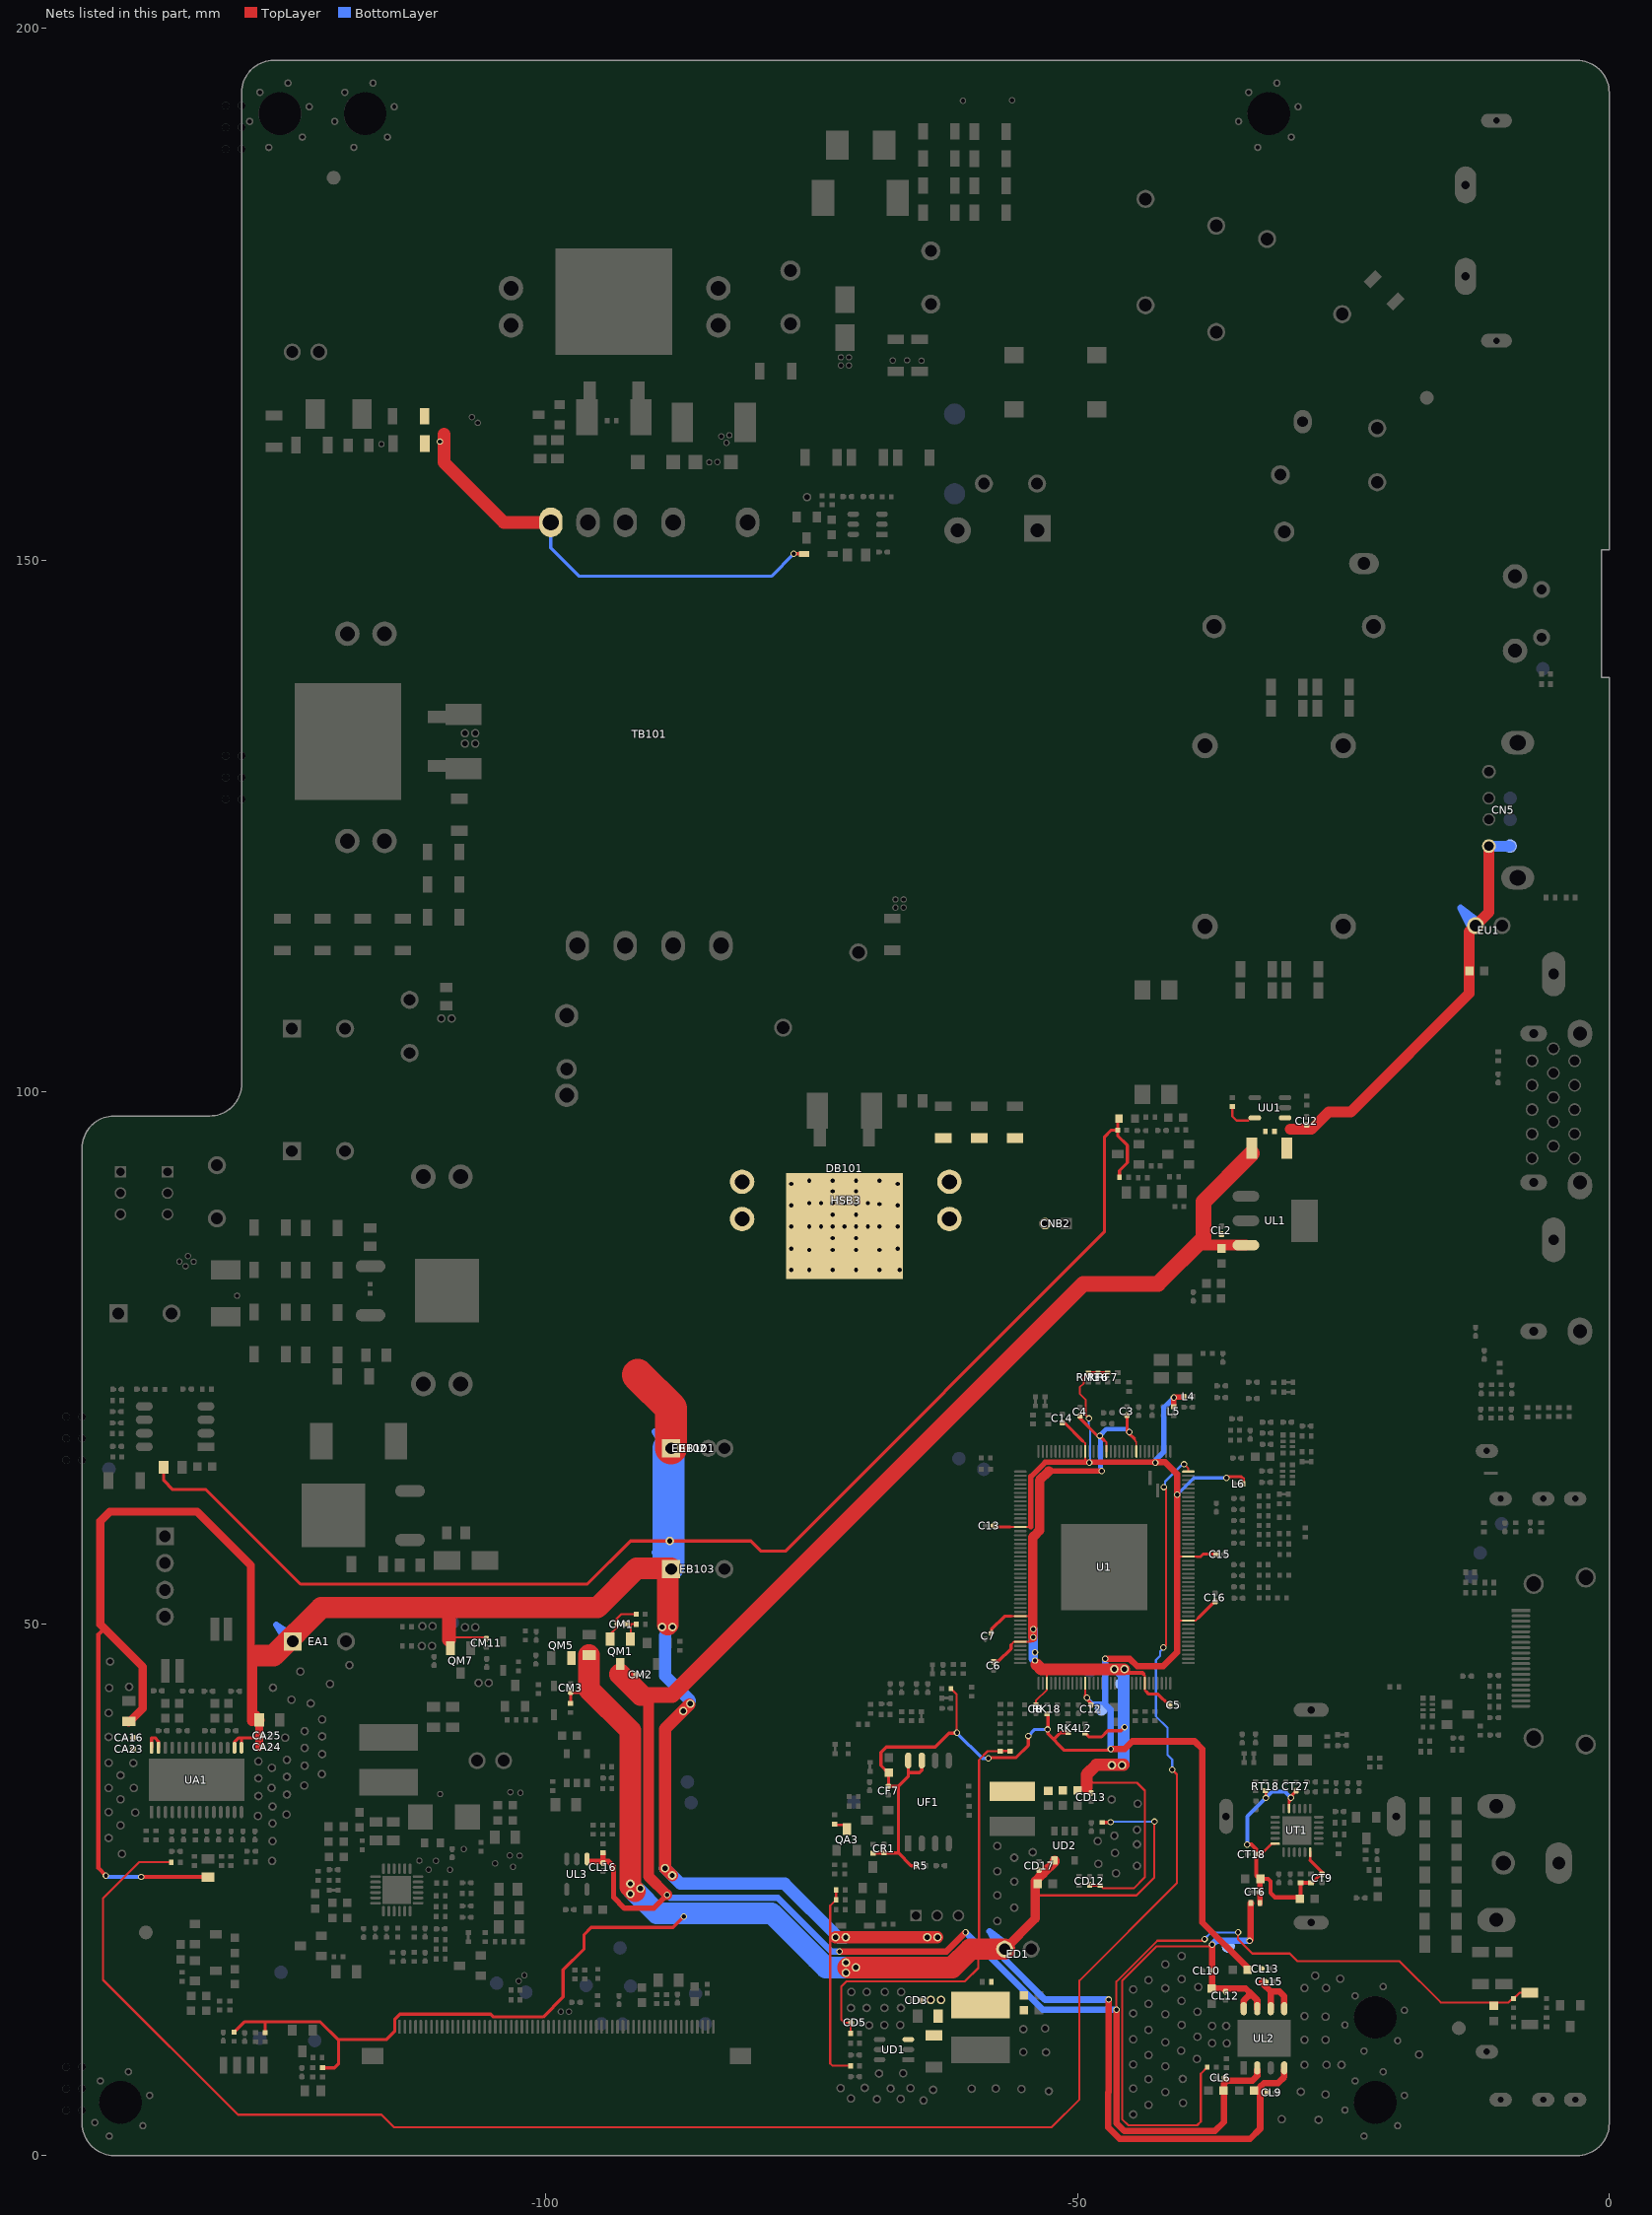
[diagram p0: the nets of this part, all layers, seen from the top]
# Altium PCB MISC86383-9.PcbDoc (part 7 of 18)
Units mm, origin at the board's own origin, x right, y up, seen from the top; angles counter-clockwise.
Board outline 143.6 x 197 mm, 2 copper layers (TopLayer, BottomLayer), stack 1.571 mm thick; 743 components, 401 nets, 2996 pads, 1077 vias.
Unrouted connection lines stored in the file: 4.

## Free pads (board coordinates)
  round 4 on Keep-Out: 0(-268.7,5) 0(-5,192)
  oval 5x4 on Keep-Out: 0(-258.2,192) 0(-15.5,5)
  round 0.7 hole 0.7 unplated: VIA5(-145.1,4.25) VIA5(-145.1,6.29) VIA5(-145.1,8.33) VIA5(-145.1,65.385) VIA5(-145.1,67.425) VIA5(-145.1,69.465) VIA5(-143.6,4.25) VIA5(-143.6,6.29) VIA5(-143.6,8.33) VIA5(-143.6,65.385) VIA5(-143.6,67.425) VIA5(-143.6,69.465) VIA5(-130.1,127.535) VIA5(-130.1,129.575) VIA5(-130.1,131.615) VIA5(-130.1,188.67) VIA5(-130.1,190.71) VIA5(-130.1,192.75) VIA5(-128.6,127.535) VIA5(-128.6,131.615) VIA5(-128.6,188.67) VIA5(-128.6,190.71) VIA5(-128.6,192.75) VIA5(-128.6,129.575)
  round 0.8 hole 0.5 paste-0.4 mask-0.4: VIA5(-141.108,29.858) VIA5(-141.108,32.293) VIA5(-141.108,34.55) VIA5(-141.108,36.923) VIA5(-141.108,39.359) VIA5(-141.108,41.616) VIA5(-141.051,43.962) VIA5(-140.972,46.448) VIA5(-139.985,31.058) VIA5(-139.985,33.494) VIA5(-139.985,35.751) VIA5(-139.865,28.364) VIA5(-139.183,44.072) VIA5(-138.789,36.901) VIA5(-138.736,34.561) VIA5(-138.613,32.249) VIA5(-127.075,31.927) VIA5(-127.036,33.802) VIA5(-127.036,35.472) VIA5(-127.036,37.052) VIA5(-125.789,34.571) VIA5(-125.75,36.447) VIA5(-125.739,27.698) VIA5(-125.699,29.573) VIA5(-125.699,31.242) VIA5(-125.699,32.822) VIA5(-125.654,43.993) VIA5(-124.511,39.281) VIA5(-124.388,32.068) VIA5(-124.349,33.943) VIA5(-124.349,35.612) VIA5(-124.349,37.192) VIA5(-123.916,42.859) VIA5(-123.084,45.51) VIA5(-122.72,34.782) VIA5(-122.68,36.657) VIA5(-122.68,38.326) VIA5(-122.68,39.907) VIA5(-122.117,42.511) VIA5(-121.062,35.866) VIA5(-121.022,37.741) VIA5(-121.022,39.41) VIA5(-121.022,40.991) VIA5(-120.288,44.34) VIA5(-118.466,46.106) VIA5(-111.658,47.904) VIA5(-111.608,49.784) VIA5(-110.693,47.904) VIA5(-110.642,49.784) VIA5(-109.83,106.921) VIA5(-108.864,106.921) VIA5(-107.607,132.766) VIA5(-107.607,133.731) VIA5(-107.594,49.67) VIA5(-106.642,132.766) VIA5(-106.642,133.731) VIA5(-106.629,49.67) VIA5(-106.324,44.45) VIA5(-105.359,44.45) VIA5(-92.05,24.587) VIA5(-92.05,25.552) VIA5(-91.11,25.095) VIA5(-89.065,49.695) VIA5(-88.794,27.021) VIA5(-88.341,57.785) VIA5(-88.111,26.338) VIA5(-88.1,49.695) VIA5(-87.084,41.796) VIA5(-86.401,42.478) VIA5(-75.425,155.943) VIA5(-72.758,20.523) VIA5(-72.268,6.335) VIA5(-71.793,20.523) VIA5(-71.78,17.17) VIA5(-71.78,18.136) VIA5(-71.305,5.352) VIA5(-71.301,13.875) VIA5(-71.279,15.377) VIA5(-70.841,17.678) VIA5(-70.01,6.361) VIA5(-69.836,13.875) VIA5(-69.814,15.377) VIA5(-69.592,12.245) VIA5(-68.869,5.301) VIA5(-68.653,7.709) VIA5(-68.17,12.263) VIA5(-68.15,13.875) VIA5(-68.128,15.377) VIA5(-67.575,6.31) VIA5(-66.663,12.263) VIA5(-66.612,5.327) VIA5(-66.608,13.875) VIA5(-66.586,15.377) VIA5(-66.396,7.734) VIA5(-65.709,6.332) VIA5(-64.478,5.173) VIA5(-64.135,20.523) VIA5(-63.805,14.63) VIA5(-63.574,6.178) VIA5(-63.17,20.523) VIA5(-62.84,14.63) VIA5(-59.95,6.275) VIA5(-57.692,6.301) VIA5(-57.541,22.035) VIA5(-57.541,24.471) VIA5(-57.541,26.728) VIA5(-57.541,29.101) VIA5(-55.947,23.314) VIA5(-55.947,25.749) VIA5(-55.947,28.006) VIA5(-55.257,6.25) VIA5(-55.103,9.738) VIA5(-55.09,11.88) VIA5(-54.216,28.516) VIA5(-53.042,11.949) VIA5(-52.967,9.703) VIA5(-52.697,6.041) VIA5(-48.108,29.566) VIA5(-48.032,27.427) VIA5(-46.787,33.477) VIA5(-46.768,36.697) VIA5(-46.535,45.744) VIA5(-46.533,30.074) VIA5(-46.482,28.448) VIA5(-46.384,26.536) VIA5(-45.803,36.697) VIA5(-45.57,45.744) VIA5(-44.77,3.862) VIA5(-44.77,6.298) VIA5(-44.77,8.555) VIA5(-44.77,10.928) VIA5(-44.77,13.363) VIA5(-44.77,15.62) VIA5(-44.405,27.228) VIA5(-44.405,29.26) VIA5(-44.405,30.632) VIA5(-44.351,33.07) VIA5(-43.326,4.747) VIA5(-43.326,7.183) VIA5(-43.326,9.44) VIA5(-43.326,11.813) VIA5(-43.326,14.248) VIA5(-43.326,16.505) VIA5(-41.739,5.956) VIA5(-41.739,8.392) VIA5(-41.739,10.649) VIA5(-41.739,13.286) VIA5(-41.739,15.722) VIA5(-41.739,17.979) VIA5(-40.254,9.848) VIA5(-40.228,14.541) VIA5(-40.208,18.748) VIA5(-40.203,12.284) VIA5(-40.195,16.592) VIA5(-40.098,7.201) VIA5(-40.073,4.944) VIA5(-38.766,9.081) VIA5(-38.71,11.176) VIA5(-38.71,13.513) VIA5(-38.645,15.833) VIA5(-37.338,10.566) VIA5(-37.338,12.192) VIA5(-36.017,12.192) VIA5(-35.966,10.54) VIA5(-30.785,3.404) VIA5(-29,5.994) VIA5(-28.651,8.534) VIA5(-28.651,10.871) VIA5(-28.651,13.106) VIA5(-28.651,15.748) VIA5(-27.635,16.916) VIA5(-27.33,3.353) VIA5(-26.67,5.74) VIA5(-26.67,10.871) VIA5(-26.67,13.056) VIA5(-26.619,15.748) VIA5(-26.568,8.534) VIA5(-25.298,16.612) VIA5(-25.171,8.522) VIA5(-17.882,9.5)
  round 0.6 hole 0.4 paste-0.4 mask-0.4: VIA5(-134.455,84.061) VIA5(-133.871,83.617) VIA5(-133.655,84.582) VIA5(-133.116,84.043) VIA5(-129.032,80.848) VIA5(-115.456,160.922) VIA5(-111.887,27.724) VIA5(-111.014,26.873) VIA5(-110.325,27.711) VIA5(-109.957,161.163) VIA5(-109.931,33.985) VIA5(-109.004,26.86) VIA5(-107.709,28.816) VIA5(-106.94,163.468) VIA5(-106.402,162.929) VIA5(-104.762,27.47) VIA5(-103.391,28.219) VIA5(-103.327,34.163) VIA5(-103.083,27.14) VIA5(-102.552,16.408) VIA5(-102.464,28.194) VIA5(-102.387,34.112) VIA5(-102.014,16.947) VIA5(-98.59,13.525) VIA5(-97.828,13.525) VIA5(-84.633,159.22) VIA5(-83.858,159.245) VIA5(-83.49,161.658) VIA5(-83.007,161.049) VIA5(-82.74,161.76) VIA5(-72.25,168.326) VIA5(-72.25,169.088) VIA5(-71.488,168.326) VIA5(-71.488,169.088) VIA5(-67.373,168.796) VIA5(-67.119,117.348) VIA5(-67.119,118.11) VIA5(-66.357,117.348) VIA5(-66.357,118.11) VIA5(-66.015,168.808) VIA5(-64.668,168.77) VIA5(-60.769,193.218) VIA5(-56.147,193.256) VIA5(-54.15,48.733) VIA5(-54.15,49.495) VIA5(-53.994,46.545) VIA5(-53.994,47.307)

## Via types
v1: diameter 0.6, hole 0.4, TopLayer to BottomLayer, tented both sides, 993 vias
v2: diameter 0.6, hole 0.4, TopLayer to BottomLayer, 65 vias
v3: diameter 0.7, hole 0.5, TopLayer to BottomLayer, tented both sides, 15 vias
v4: diameter 0.8, hole 0.5, TopLayer to BottomLayer, tented both sides, 4 vias

## Nets (pads, with @x,y where several pads share a name; then routed paths per layer and width w, separated by ;. In a path a pad name is that pad's centre, name@x,y a point inside that pad or via, vN(x,y) a via of type N, cw(c..) or ccw(c..) an arc to the next point about the centre after c; other vN are vias at no path point)
1.15V_STB: 1.15V_STB.1 C3.2@-45.337,69.569 C3.2@-45.337,69.744 C4.2@-49.757,69.68 C4.2@-49.757,69.505 C5.2@-41.206,42.333 C5.2@-41.381,42.333 C6.2@-57.891,46.297 C6.2@-57.891,46.472 C7.2@-58.079,49.149 C7.2@-58.203,49.025 C8.2@-53.91,42.228 C8.2@-53.91,42.403 CD10.2 CD12.2@-48.854,25.57 CD12.2@-48.854,25.395 CD13.2@-48.717,33.943 CD13.2@-48.717,34.118 CD14.2 CD15.2 L2.1 LD2.1 pad.VIA5@-45.57,45.744 pad.VIA5@-45.803,36.697 pad.VIA5@-46.535,45.744 pad.VIA5@-46.768,36.697 pad.VIA5@-53.994,46.545 pad.VIA5@-53.994,47.307 pad.VIA5@-54.15,48.733 pad.VIA5@-54.15,49.495 RD9.1 U1.55 U1.62 U1.113 U1.119 U1.127 U1.150 | length 103.6
  TopLayer w0.178: -56.259,48 -55.947,48.313 -54.344,48.313 ; -56.246,50.715 -56.244,50.713 -54.199,50.713 ; C8.2@-53.91,42.403 -53.91,42.749 -52.871,43.788 -52.871,45.343 ; -47.458,67.251 -47.271,67.063 U1.62@-47.271,66.213 ; -44.661,67.311 -44.471,67.121 U1.55@-44.471,66.213 ; -43.811,45.303 -43.671,45.163 -43.671,43.758 -43.518,43.605
  TopLayer w0.203: CD15.2@-51.372,34.33 CD15.2@-51.318,34.383 ; CD10.2@-49.974,34.323 CD10.2@-49.947,34.296 ; CD12.2@-48.854,25.395 RD9.1@-47.865,25.395 -47.591,25.121 -44.717,25.121 -43.663,26.175 -43.663,34.315 -44.399,35.052 -48.565,35.052 -48.768,35.255
  TopLayer w0.305: C7.2@-58.079,49.149 -58.079,49.495 -56.859,50.715 -56.246,50.715 ; C6.2@-57.891,46.472 -57.437,46.472 -56.259,47.65 -56.259,48 ; C4.2@-49.757,69.505 -49.757,69.312 v1@-48.112,67.667 ; L2.1@-49.122,39.552 -48.931,39.361 -47.734,39.361 -47.163,39.933 -45.919,39.933 v1(-45.568,40.284) ; v1@-47.918,67.667 -47.502,67.251 ; -45.337,69.162 C3.2@-45.337,69.569 ; -45.336,69.268 -45.336,68.068 v1@-45.206,67.938 ; v1(-45.11,68.034) v1@-45.206,67.938 ; -44.629,67.361 v1@-45.206,67.938 ; -43.518,43.605 -43.3,43.387 -42.435,43.387 C5.2@-41.381,42.333
  TopLayer w0.381: pad.VIA5@-45.629,45.711 -45.615,45.698 -45.302,45.384 -43.892,45.384 -43.811,45.303
  TopLayer w0.508: -52.699,64.36 v1(-47.725,64.36)
  TopLayer w0.889: pad.VIA5@-54.199,48.683 -54.199,48.733 -54.199,49.495 -54.199,50.713 -54.199,58.173 -54.085,58.287 -54.048,58.287 -53.564,58.771 -53.564,59.364 -53.564,63.495 -52.699,64.36
  TopLayer w1.143: -53.841,46.162 -53.39,45.711 -46.535,45.711 pad.VIA5@-45.629,45.711 ; -49.136,34.604 -49.136,35.827 -48.222,36.741 -46.768,36.741 -45.803,36.741 pad.VIA5@-45.663,36.741
  BottomLayer w0.457: v1(-47.725,64.36) -47.826,64.462 -47.826,67.674 -47.826,67.772 -47.293,68.305 -45.382,68.305 v1(-45.11,68.034)
  BottomLayer w0.889: pad.VIA5@-54.15,46.701 -54.15,47.307 pad.VIA5@-54.15,48.733 pad.VIA5@-54.15,49.495
  BottomLayer w1.143: -45.923,45.466 -45.885,45.428 -45.663,45.205 -45.663,44.348 -45.663,40.284 pad.VIA5@-45.663,36.785
  other v1: -47.911,67.674
3V3_STB: 3V3_STB.1 C12.2@-48.728,42.228 C12.2@-48.728,42.403 C13.2@-57.853,59.212 C13.2@-58.028,59.212 C14.2@-51.435,68.885 C14.2@-51.435,69.06 C15.2@-36.826,56.54 C15.2@-37.001,56.54 C16.2@-37.059,52.051 C16.2@-37.059,52.226 CF7.1 CF10.2 CL13.1 CL14.1 CL15.1 CR1.2@-68.191,28.441 CR1.2@-68.191,28.616 L4.1 L5.1 L6.1 R5.2 RF6.2 RF7.2 RF14.1 RK4.2 RK18.2 RM3.1 RR5.2 U1.11 U1.26 U1.67 U1.92 U1.136 UF1.7 UF1.8 UL2.5 UL2.6 | length 190.8
  TopLayer w0.178: -56.348,59.11 -56.345,59.113 -54.412,59.113 ; -49.505,67.183 -49.271,66.949 U1.67@-49.271,66.213 -49.271,65.292 ; -49.271,43.32 U1.136@-49.271,44.413 ; RM3.1@-48.969,73.581 -48.987,73.581 -49.41,73.158 -49.41,72.631 -49.785,72.256 -49.785,71.636 -49.206,71.057 -49.206,69.58 v1(-48.93,69.305) ; -40.617,50.313 U1.11@-39.571,50.313 -38.881,50.313 -38.653,50.541 ; -40.371,56.313 -38.768,56.313
  TopLayer w0.203: RF14.1@-61.907,43.901 -61.366,43.361 -61.366,39.776 -61.341,39.751 v1@-61.328,39.738
  TopLayer w0.254: -38.768,56.313 -38.412,56.313 -38.17,56.555 C15.2@-37.076,56.555
  TopLayer w0.305: RR5.2@-69.207,28.415 -68.216,28.415 CR1.2@-68.191,28.441 -66.893,28.441 ; UF1.8@-65.916,37.142 -65.916,35.965 ; R5.2@-65.137,27.254 -65.636,27.254 -66.858,28.476 -66.84,28.494 -66.84,34.688 ; UF1.7@-64.646,37.142 -64.632,37.128 -64.632,36.215 -64.853,35.994 -65.887,35.994 -65.916,35.965 ; v1@-61.328,39.738 -61.29,39.7 -61.328,39.7 -62.078,39.7 -63.378,38.4 -67.988,38.4 -68.484,37.904 -68.484,36.672 -67.787,35.975 -67.778,35.975 CF10.2@-67.755,35.997 -67.755,34.749 CF7.1@-67.783,34.721 -66.873,34.721 -66.84,34.688 ; v1(-58.369,37.338) -58.445,37.414 -58.369,37.414 -55.778,37.414 -54.62,38.572 v1(-54.62,39.45) ; C13.2@-57.853,59.212 -57.752,59.11 -56.348,59.11 ; RK18.2@-52.779,41.527 -52.779,40.059 -52.779,39.643 -51.24,38.104 v1@-47.088,38.104 ; -52.195,39.158 -51.592,39.762 RK4.2@-50.874,39.762 ; C14.2@-51.435,68.885 -51.201,68.885 -49.505,67.188 -49.505,67.183 ; v1@-49.249,43.298 -49.249,43.056 -49.186,42.994 -48.728,42.536 C12.2@-48.728,42.403 C12.2@-48.728,42.228 ; RM3.1@-48.901,73.593 RF6.2@-48.062,73.593 RF7.2@-47.147,73.593 RF7.2@-47.071,73.593 ; C12.2@-48.713,42.417 C12.2@-48.688,42.392 ; C12.2@-48.677,42.228 C12.2@-48.677,42.381 ; -38.653,50.541 -37.143,52.051 C16.2@-37.059,52.051 ; v1@-35.956,63.68 v1(-36.005,63.729) -35.903,63.83 -34.595,63.83 -34.385,63.62 L6.1@-34.385,63.17 ; -66.84,34.688 -65.916,35.613 -65.916,35.965
  TopLayer w0.508: -54.39,59.113 -54.39,63.837 -53.041,65.185 -48.893,65.185 v1@-42.784,65.185 ; L5.1@-40.959,70.58 -40.959,71.235 v1(-40.93,71.264) -40.895,71.299 -40.191,71.299 L4.1@-40.164,71.326
  TopLayer w0.61: v1(-47.401,46.715) -45.093,46.715 -44.385,46.007 -41.951,46.007 -40.628,47.329 -40.628,62.154 -40.628,64.066 -41.743,65.181 -42.683,65.181 v1@-42.784,65.181 ; v1@-46.863,38.231 -45.562,38.231 -44.851,38.942 -38.979,38.942 -38.259,38.222 -38.259,21.921 -33.99,17.652 CL14.1@-33.99,17.475 ; -32.66,16.358 -32.66,16.251 -32.572,16.164 -32.485,16.076 -31.826,15.418 ; UL2.6@-31.826,13.806 -31.826,15.418 ; UL2.5@-30.556,13.806 -30.556,14.961 -31.013,15.418 -31.826,15.418
  BottomLayer w0.178: v1(-48.93,69.305) -48.93,68.488 -48.792,68.35 v1@-48.792,65.257
  BottomLayer w0.305: v1@-61.341,39.726 -58.953,37.338 v1(-58.369,37.338) ; v1(-54.62,39.45) -54.012,40.059 v1(-52.806,40.059) ; v1(-49.123,43.056) -48.608,42.541 -47.752,42.541 3V3_STB.1@-47.511,42.541 ; v1(-40.64,62.154) -39.065,63.729 v1(-36.005,63.729)
  BottomLayer w0.508: v1(-42.683,65.155) -42.683,65.371 -41.862,66.192 -41.862,70.332 v1(-40.93,71.264)
  BottomLayer w0.61: v1@-47.387,46.7 v1(-47.401,46.715) -47.401,42.431 -47.367,42.397 -46.888,41.918 -46.888,38.227 -46.876,38.214 -46.863,38.202 v1(-46.863,38.227)
  other v1: -61.328,39.764 -48.893,65.155
3V3_TUN: CT2.2 CT5.2 CT6.1 CT9.1 CT18.2@-33.189,28.323 CT18.2@-33.364,28.323 CT27.1 LT1.1 LT2.2 LT12.2 RT18.1 UT1.11 UT1.18 UT1.24 | length 30.2
  TopLayer w0.203: RT18.1@-32.344,34.299 -32.293,34.248 v1(-32.293,33.619) ; UT1.11@-30.11,32.62 -30.11,33.263 -30.071,33.301
  TopLayer w0.229: CT18.2@-33.189,28.323 -32.741,28.323 -31.744,29.32 UT1.18@-31.41,29.32 ; UT1.24@-28.11,28.52 -28.11,27.771 -28.102,27.764
  TopLayer w0.305: -30.071,33.301 -30.071,33.638 -29.998,33.711 v1@-29.931,33.778 ; v1(-29.931,33.644) v1@-29.931,33.778 ; CT27.1@-29.436,34.273 v1@-29.931,33.778 ; -28.102,27.764 CT9.1@-26.997,26.659 ; LT1.1@-27.922,25.638 -27.122,26.437 CT9.1@-27.072,26.487
  TopLayer w0.381: v1(-34.033,29.245) -33.647,29.245 -33.189,28.787 CT18.2@-33.189,28.323 -33.189,26.314 -32.887,26.012 -32.838,26.012 CT5.2@-32.811,26.012 -32.065,26.012 -31.836,25.783 -31.836,24.691 -31.421,24.277 -29.302,24.277 -29.27,24.309 -29.029,24.549 LT2.2@-29.029,25.638 LT1.1@-28.064,25.638 LT1.1@-27.922,25.638 ; CT9.1@-27.072,26.487 CT9.1@-26.997,26.487
  TopLayer w0.508: LT12.2@-32.838,23.726 -32.838,24.767 CT5.2@-32.838,26.012
  BottomLayer w0.381: v1(-34.033,29.245) -34.033,31.88 v1(-32.293,33.619) -31.689,34.224 -30.511,34.224 v1(-29.931,33.644)
3V3_TUNER: 3V3_TUNER.1 CL10.2@-37.421,17.374 CL10.2@-37.596,17.374 CL11.1 CL12.2@-36.068,15.262 CL12.2@-36.068,15.437 LT12.1 RL5.2 UL2.7 UL2.8 | length 54.7
  TopLayer w0.203: RL5.2@-37.795,8.306 -38.405,7.696 -38.405,3.175 -38.748,2.832 -45.22,2.832 -45.806,3.419 -45.806,16.423 -42.569,19.66 -37.519,19.66 v1(-37.338,19.841)
  TopLayer w0.508: LT12.1@-33.701,23.738 LT12.1@-33.688,23.726
  TopLayer w0.61: v1(-37.338,19.841) -37.338,17.374 -37.338,15.743 CL11.1@-37.389,15.692 -36.068,15.692 -34.184,15.692 -33.706,15.215 ; UL2.8@-34.366,13.806 -34.366,14.554 -33.706,15.215 ; v1(-33.817,20.181) -33.714,20.284 -33.714,23.7 LT12.1@-33.688,23.726 ; UL2.7@-33.096,13.806 -33.096,14.605 -33.706,15.215
  BottomLayer w0.61: v1(-37.338,19.841) -37.33,19.841 -36.99,20.181 -35.82,20.181 v1(-33.817,20.181)
5V_M: CL1.2 CL2.2@-36.449,86.566 CL2.2@-36.449,86.741 CL6.2@-36.3,7.315 CL6.2@-36.125,7.315 CL7.2 CL16.1 CM2.1 CO77.1 F2.1 FU1.2 QM1.D RL50.1 RO2.2 RO6.1 RU4.2 UL1.3 UL2.2 UL3.1 UU1.5 | length 247
  TopLayer w0.203: v1(-46.339,13.705) -46.339,16.356 -42.49,20.206 -38.2,20.206 v1(-38.053,20.353) ; RU4.2@-35.433,98.635 -35.433,97.714 -35.046,97.327 -33.927,97.327 ; v1(-34.899,20.973) -34.899,20.347 -33.551,18.999 -30.033,18.999 -29.296,18.263 -19.699,18.263 -15.828,14.391 -10.846,14.391 -9.465,14.391 -9.051,14.805 -8.992,14.864 RO6.1@-8.992,14.746 -8.425,15.313 RO2.2@-7.468,15.313
  TopLayer w0.508: UL3.1@-96.012,27.648 CL16.1@-94.628,27.648 ; RL50.1@-94.628,28.468 CL16.1@-94.628,27.648 ; CL16.1@-94.615,27.539 -94.628,27.552 CL16.1@-94.628,27.648 ; CL16.1@-94.615,27.648 -94.094,27.648 -93.624,27.178 -93.624,24.282 -92.596,23.254 -89.852,23.254 v1(-88.595,24.511)
  TopLayer w0.61: v1(-72.384,19.177) -62.332,19.177 v1(-60.528,20.98) ; v1(-46.339,13.705) -46.339,3.039 -45.599,2.299 -37.071,2.299 -36.22,3.15 -36.22,6.096 -36.22,6.756 -35.981,6.996 -35.928,7.048 -33.541,7.048 -33.096,7.493 UL2.2@-33.096,8.038
  TopLayer w1.016: -91.078,43.313 -90.33,42.566 -90.33,26.246 v1(-88.595,24.511) ; -38.713,85.598 -36.449,85.598 UL1.3@-34.163,85.598
  TopLayer w1.5: -91.078,43.313 -88.098,43.313 -49.445,81.966 -42.418,81.966 -38.151,86.233 -38.151,89.687 FU1.2@-33.603,94.235
  TopLayer w2.032: -93.003,45.239 -92.262,44.497 -92.174,44.41 -91.078,43.313
  BottomLayer w0.203: v1(-38.053,20.353) -37.433,20.973 v1(-34.899,20.973)
  BottomLayer w0.61: v1(-88.595,24.511) -88.316,24.232 -78.181,24.232 -73.127,19.177 v1(-72.384,19.177) ; v1(-60.528,20.98) -53.264,13.716 v1@-46.339,13.716
5V_MOS_G: CM1.2@-92.65,49.974 CM1.2@-92.475,49.975 QM1.G RM2.2 | length 2.4
  TopLayer w0.203: CM1.2@-92.475,49.975 -91.999,49.975 ; QM1.G@-92.053,48.571 -91.999,48.625 -91.999,49.975 ; RM2.2@-91.484,49.962 -91.497,49.975 -91.999,49.975
5V_STB: 5V_STB.1 CD5.2@-71.169,12.49 CD5.2@-71.344,12.49 CD7.2 CD9.2 CD16.2 CD17.2@-53.619,26.804 CD17.2@-53.619,26.979 CL8.2 CL9.2@-32,5.944 CL9.2@-32.175,5.944 CM1.1 CM3.2@-97.665,43.538 CM3.2@-97.665,43.713 CM5.2 DK6.K ED1.1 LD1.2 pad.VIA5@-70.841,17.678 pad.VIA5@-71.78,17.17 pad.VIA5@-71.78,18.136 pad.VIA5@-91.11,25.095 pad.VIA5@-92.05,24.587 pad.VIA5@-92.05,25.552 QM1.S QM5.S RD3.2 RD7.2 RK1.2 RK13.1 RK15.1 RM1.2 RM5.2 RV12.2 RV13.2 UD2.4 UL2.4 | length 246.9
  TopLayer w0.203: QM1.S@-93.953,48.571 -93.953,48.998 -93.325,49.626 CM1.1@-93.325,49.974 -93.332,49.981 -93.332,50.482 -92.913,50.902 RM1.2@-91.497,50.902 ; RD3.2@-71.343,11.474 CD5.2@-71.344,12.49 -71.926,12.49 -72.212,12.776 -72.212,15.875 -71.704,16.383 -60.579,16.383 -59.334,17.628 -59.334,18.684 -60.056,19.406 -59.258,20.203 -59.258,37.197 -58.444,38.011 -57.277,38.011 RV13.2@-57.277,38.031 ; RV13.2@-57.247,38.04 -56.35,38.04 RV12.2@-56.333,38.04 ; -53.975,24.308 -53.823,24.46 -44.444,24.46 -42.774,26.13 v1(-42.774,31.394)
  TopLayer w0.305: RK13.1@-129.316,11.591 -128.342,12.565 -126.39,12.565 ; RK15.1@-126.39,11.55 -126.39,12.565 ; RK1.2@-121.006,8.248 -119.882,8.248 -119.482,8.649 -119.482,10.846 ; RM5.2@-97.665,42.508 CM3.2@-97.665,43.538 -96.581,43.538 ; v1(-87.008,22.479) -88.041,21.445 -95.722,21.445 -96.406,20.762 -96.406,19.418 -98.369,17.455 -98.369,14.913 -100.251,13.032 -100.677,13.032 -100.681,13.028 -104.914,13.028 -105.172,13.286 -113.737,13.286 -114.195,12.828 -114.195,11.714 -115.012,10.897 -119.431,10.897 -119.482,10.846 ; RD7.2@-47.689,31.322 -46.91,31.322 v1(-46.888,31.344) ; -126.39,12.565 -121.201,12.565 -119.482,10.846
  TopLayer w0.61: v1(-47.076,14.661) -47.076,5.949 -47.097,5.928 -47.097,2.624 -46.035,1.562 -33.769,1.562 -32.817,2.515 -32.817,6.096 -32.817,6.452 -32.461,6.807 -31.14,6.807 -30.556,7.391 UL2.4@-30.556,8.038
  TopLayer w0.889: ED1.1@-56.851,19.406 -53.975,22.281 -53.975,24.308 -53.975,25.552 -53.975,25.781 -53.973,25.783 -53.286,26.47 -53.198,26.558 -52.149,27.607 UD2.4@-52.149,27.757
  TopLayer w2.032: CM5.2@-95.936,47.053 -95.936,43.85 -92.062,39.976 -92.062,25.552 -92.062,25.286 -91.707,24.93 -91.611,24.835 ; -71.552,17.678 pad.VIA5@-70.841,17.678 -61.783,17.678 -60.056,19.406 ED1.1@-56.851,19.406
  BottomLayer w0.203: v1(-46.888,31.344) -46.838,31.394 v1(-42.774,31.394)
  BottomLayer w0.305: v1@-47.016,31.344 v1(-46.888,31.344)
  BottomLayer w0.61: ED1.1@-56.851,19.406 -56.851,18.446 -53.061,14.656 v1@-47.076,14.656
  BottomLayer w2.032: -91.796,25.019 -91.707,24.93 -91.491,24.714 -89.56,22.784 -87.008,22.784 -78.781,22.784 -74.557,18.56 -73.675,17.678 -71.78,17.678 -71.349,17.678
5V_USB: CN5.1@-11.31,123.13 CU1.2 CU2.1 EU1.1 F2.2 FU1.1 USB_5V.1 UU1.1 | length 38.8
  TopLayer w1.016: -30.003,96.502 -28.448,96.502 -27.984,96.502 -27.949,96.537 -26.365,98.12 -24.308,98.12 -13.152,109.276 CU1.2@-13.152,111.379 -13.152,115.072 EU1.1@-12.578,115.646 -11.31,116.915 CN5.1@-11.31,123.13
  BottomLayer w1.016: CN5.1@-11.31,123.13 USB_5V.1@-9.31,123.13
12V: CA16.2@-138.766,39.278 CA16.2@-138.941,39.278 CA23.2@-138.766,38.212 CA23.2@-138.941,38.212 CA24.2@-126.483,38.427 CA24.2@-126.658,38.427 CA25.2@-126.483,39.494 CA25.2@-126.658,39.494 CA31.2 CA32.2 CD1.2 CD2.1 CD3.2@-64.7,14.605 CD3.2@-64.875,14.605 CM11.2@-105.588,48.447 CM11.2@-105.588,48.622 CNB2.2 DB101.2 EA1.1@-123.798,48.336 EB101.1@-88.212,66.497 EB102.1@-88.212,66.497 EB103.1@-88.212,55.143 HSB3.1 HSB3.2 HSB3.3 HSB3.4 pad.VIA5@-62.84,14.63 pad.VIA5@-63.17,20.523 pad.VIA5@-63.805,14.63 pad.VIA5@-64.135,20.523 pad.VIA5@-71.793,20.523 pad.VIA5@-72.758,20.523 pad.VIA5@-86.401,42.478 pad.VIA5@-87.084,41.796 pad.VIA5@-88.1,49.695 pad.VIA5@-88.111,26.338 pad.VIA5@-88.341,57.785 pad.VIA5@-88.794,27.021 pad.VIA5@-89.065,49.695 QM7.S RA3.1 RA16.1 RA19.2 RB128.2 RB129.2 RB131.2 RB135.1 RB158.2 RB165.2 RB816.1 RD1.1 UA1.15 UA1.16 UA1.27 UA1.28 UD1.3 | length 367.1
  TopLayer w0.203: -108.925,48.73 -105.696,48.73 CM11.2@-105.588,48.622 ; RA16.1@-72.705,24.04 -73.254,23.491 -73.254,21.438 -73.254,8.661 -73.027,8.435 RD1.1@-71.345,8.435
  TopLayer w0.254: RA16.1@-72.705,24.04 RA19.2@-72.705,24.98
  TopLayer w0.3: RB816.1@-135.931,64.706 -135.931,63.477 -135.075,62.621 -131.953,62.621 -123.063,53.731 -96.087,53.731 -92.033,57.785 pad.VIA5@-88.341,57.785 -80.705,57.785 -79.747,56.827 -77.473,56.827 -47.473,86.828 -47.473,95.758 -46.812,96.418 RB158.2@-46.221,96.418 ; RB131.2@-46.102,97.511 -46.221,97.392 RB158.2@-46.221,96.418 ; RB135.1@-46.043,91.973 -46.043,92.615 -45.3,93.358 -45.3,94.983 -46.221,95.904 RB158.2@-46.221,96.418
  TopLayer w0.305: UA1.28@-137.07,38.341 -137.07,39.257 -137.092,39.278 -136.761,39.278 -136.42,38.937 UA1.27@-136.42,38.341 ; UA1.16@-129.27,38.341 -129.27,38.863 -128.855,39.278 -128.57,39.278 ; UA1.15@-128.62,38.341 -128.62,39.228 -128.57,39.278 ; -126.945,39.278 -128.57,39.278
  TopLayer w0.381: -141.519,49.559 -142.076,49.002 -142.076,27.021 v1(-141.366,26.311) ; v1(-138.06,26.199) -131.813,26.199 RA3.1@-131.783,26.17
  TopLayer w0.762: CA31.2@-139.238,40.7 -137.904,42.033 -137.904,45.944 -141.519,49.559 -141.886,49.925 -141.886,59.665 -141.009,60.541 -132.779,60.541 -127.724,55.486 -127.724,46.965 -127.622,46.863 ; -126.945,38.414 -126.945,39.278 CA32.2@-126.945,40.955
  TopLayer w1.016: -127.622,40.881 -127.622,46.863 -127.47,47.015 ; CA32.2@-127.338,41.348 CA32.2@-126.945,40.955
  TopLayer w1.143: pad.VIA5@-88.111,26.338 pad.VIA5@-88.794,27.021 -88.794,40.102 pad.VIA5@-86.486,42.409 ; pad.VIA5@-72.758,20.523 pad.VIA5@-71.793,20.523 pad.VIA5@-64.135,20.523 pad.VIA5@-63.17,20.523
  TopLayer w1.27: -127.47,47.015 -127.089,47.015 ; -109.436,51.524 -109.11,51.198 -109.11,48.472
  TopLayer w2.032: -127.089,47.015 -125.603,47.015 -121.094,51.524 -109.436,51.524 -95.136,51.524 -91.44,55.22 -88.25,55.22 -88.519,54.951 -88.519,49.916
  TopLayer w3: -91.351,73.393 -88.212,70.255 EB101.1@-88.212,66.497
  BottomLayer w0.3: EB103.1@-88.212,55.143 EB103.1@-88.212,55.727
  BottomLayer w0.381: v1(-141.366,26.311) -141.254,26.199 v1(-138.06,26.199)
  BottomLayer w1.143: pad.VIA5@-88.794,27.021 pad.VIA5@-88.111,26.338 -87.338,25.565 -77.529,25.565 -72.487,20.523 pad.VIA5@-71.793,20.523 ; -88.786,48.895 -88.786,45.115 pad.VIA5@-86.452,42.781
  BottomLayer w3: EB103.1@-88.466,55.45 -88.466,55.886 EB101.1@-88.466,66.497
  other v1: -76.918,83.261 -75.218,83.26 -73.018,83.261 -70.818,83.261 -68.618,83.261 -66.719,83.261 -75.218,85.161 -73.018,85.161 -70.818,85.161 -68.618,85.161 -76.918,85.261 -66.918,85.261 -73.018,86.261 -70.818,86.261 -76.919,87.361 -75.218,87.361 -74.118,87.361 -73.018,87.361 -71.918,87.361 -70.818,87.361 -69.718,87.361 -68.618,87.361 -66.919,87.361 -73.018,88.461 -70.818,88.461 -76.918,89.361 -66.918,89.361 -70.818,89.461 -68.618,89.461 -75.218,89.561 -74.119,89.561 -73.018,89.561 -71.918,89.561 -69.718,89.561 -73.018,90.661 -70.818,90.661 -76.918,91.361 -66.918,91.361 -75.218,91.661 -73.018,91.66 -70.818,91.66 -68.618,91.661
12V-OVP: DB112.A pad.VIA5@-109.957,161.163 RB114.2 RB115.2 TB101.6 | length 43.3
  TopLayer w0.3: v2(-76.683,150.609) DB112.A@-75.721,150.609
  TopLayer w1.2: -109.588,161.849 -109.588,161.163 -109.588,159.207 -103.948,153.567 TB101.6@-99.528,153.567
  BottomLayer w0.3: TB101.6@-99.528,153.567 -99.528,151.179 -96.85,148.501 -78.791,148.501 v2(-76.683,150.609) v2@-76.568,150.609
AC_OFF_DET: QA3.C RR6.2 | length 1.6
  TopLayer w0.203: RR6.2@-72.847,31.173 -72.764,31.09 -71.73,31.09 -71.683,31.043 QA3.C@-71.683,30.695
AMP-LO: RA21.1 U1.46 | length 180.8
  TopLayer w0.178: U1.46@-39.571,64.313 -39.571,64.603
  TopLayer w0.203: RA21.1@-135.223,27.584 -138.234,27.584 -141.632,24.187 -141.632,16.52 -128.947,3.835 -115.459,3.835 -114.283,2.659 -52.443,2.659 -49.815,5.287 -49.815,16.437 -40.646,25.606 -40.646,35.833 v1(-41.097,36.284) ; v1(-41.923,47.765) -41.662,48.026 -41.662,62.642 v1(-41.872,62.852) ; v1(-39.967,64.999) -39.571,64.603
  BottomLayer w0.203: v1(-41.923,47.765) -41.897,47.739 -42.224,47.412 -42.224,46.987 -42.621,46.59 -42.621,41.298 -41.531,40.208 -41.531,37.67 -41.097,37.236 v1(-41.097,36.284) ; v1(-41.872,62.852) -41.77,62.852 -41.77,63.373 -40.145,64.999 v1(-39.967,64.999)